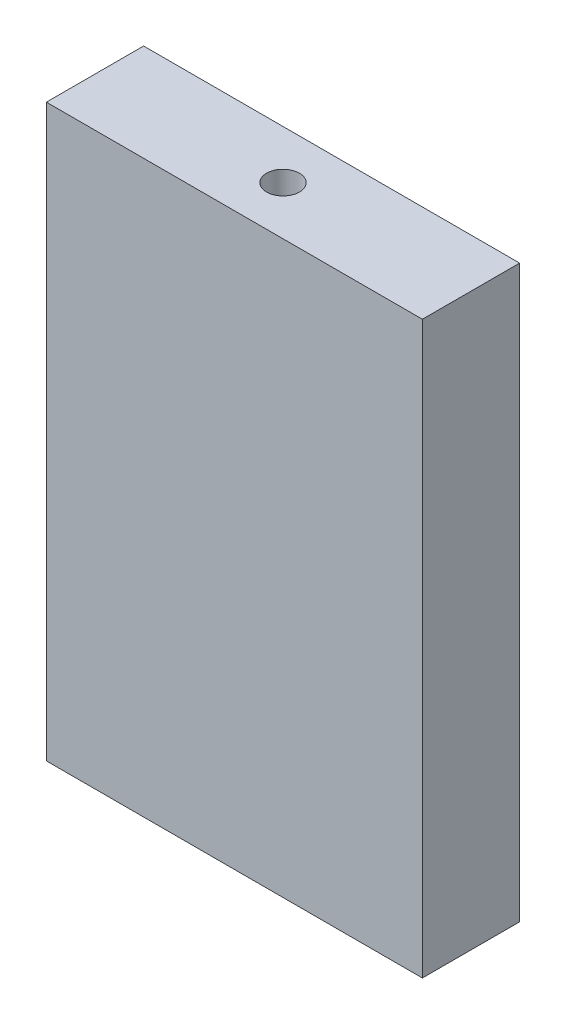
SolidWorks part; units mm, degrees
ref_plane "Front Plane" through (0, 0, 0) normal (0, 0, 1) x (1, 0, 0)
ref_plane "Top Plane" through (0, 0, 0) normal (0, 1, 0) x (1, 0, 0)
ref_plane "Right Plane" through (0, 0, 0) normal (1, 0, 0) x (0, 0, -1)
sketch "Sketch1" plane through (0, 0, 0) normal (0, 0, 1) x (1, 0, 0)
  line L1 (58, 88) -> (-58, 88)
  line L2 (58, 88) -> (58, -88)
  line L3 (58, -88) -> (-58, -88)
  line L4 (-58, 88) -> (-58, -88)
  line L5 (58, 88) -> (-58, -88) construction
  line L6 (58, -88) -> (-58, 88) construction
  point P0 (0, 0)
  dimension "D1" = 116
  dimension "D2" = 176
extrude "Boss-Extrude1" add sketch "Sketch1" along normal blind 30
sketch "Sketch3" plane through (0, 88, 0) normal (0, 1, 0) x (1, 0, 0)
  line L0 (-58, -30) -> (-58, 0) construction
  circle A0 centre (0, -15) radius 5.055
  point P4 (-58, -15)
  dimension "D1" = 10.11
extrude "Cut-Extrude1" cut sketch "Sketch3" against normal through all
